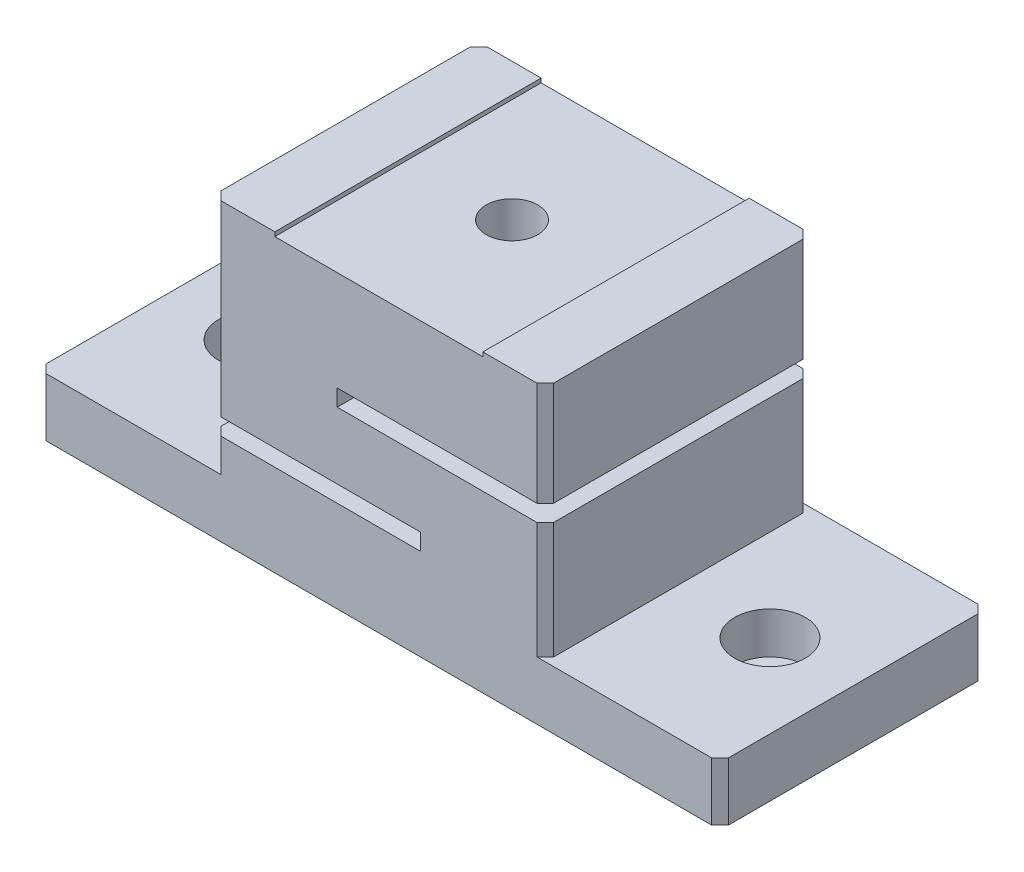
SolidWorks part; units mm, degrees
ref_plane "Front Plane" through (0, 0, 0) normal (0, 0, 1) x (1, 0, 0)
ref_plane "Top Plane" through (0, 0, 0) normal (0, 1, 0) x (1, 0, 0)
ref_plane "Right Plane" through (0, 0, 0) normal (1, 0, 0) x (0, 0, -1)
sketch "Sketch1" plane through (0, 0, 0) normal (0, 1, 0) x (1, 0, 0)
  line L1 (-41, -16) -> (41, -16)
  line L2 (-41, -16) -> (-41, 16)
  line L3 (-41, 16) -> (41, 16)
  line L4 (41, -16) -> (41, 16)
  line L5 (-41, -16) -> (41, 16) construction
  line L6 (-41, 16) -> (41, -16) construction
  point P0 (0, 0)
  dimension "D1" = 82
  dimension "D2" = 32
extrude "Boss-Extrude1" add sketch "Sketch1" along normal blind 7
sketch "Sketch2" plane through (0, 7, 0) normal (0, 1, 0) x (1, 0, 0)
  line L0 (41, 16) -> (-41, 16) construction
  line L1 (-20, -16) -> (20, -16)
  line L2 (-20, -16) -> (-20, 16)
  line L3 (-20, 16) -> (20, 16)
  line L4 (20, -16) -> (20, 16)
  line L5 (-20, -16) -> (20, 16) construction
  line L6 (-20, 16) -> (20, -16) construction
  point P0 (0, 0)
  dimension "D1" = 40
extrude "Boss-Extrude2" add sketch "Sketch2" along normal blind 28.5
sketch "Sketch3" plane through (0, 7, 0) normal (0, 1, 0) x (1, 0, 0)
  line L0 (20, -16) -> (41, -16) construction
  line L1 (41, -16) -> (41, 16) construction
  line L2 (-41, -16) -> (-20, -16) construction
  line L3 (-41, 16) -> (-41, -16) construction
  circle A0 centre (31, 0) radius 2.1
  circle A1 centre (-31, 0) radius 2.1
  dimension "D1" = 4.2
  dimension "D2" = 4.2
  dimension "D3" = 16
  dimension "D4" = 10
  dimension "D5" = 16
  dimension "D6" = 10
extrude "Cut-Extrude1" cut sketch "Sketch3" against normal blind 28.5
sketch "Sketch4" plane through (0, 7, 0) normal (0, 1, 0) x (1, 0, 0)
  circle A0 centre (-31, 0) radius 4.25
  circle A1 centre (31, 0) radius 4.25
  dimension "D1" = 8.5
  dimension "D2" = 8.5
extrude "Cut-Extrude2" cut sketch "Sketch4" against normal blind 5
sketch "Sketch5" plane through (0, 0, -16) normal (0, 0, -1) x (-1, 0, 0)
  line L0 (20, 35.5) -> (20, 7) construction
  line L1 (-5, 13) -> (45, 13)
  line L2 (-5, 13) -> (-5, 11)
  line L3 (-5, 11) -> (45, 11)
  line L4 (45, 13) -> (45, 11)
  line L5 (-5, 13) -> (45, 11) construction
  line L6 (-5, 11) -> (45, 13) construction
  line L7 (20, 7) -> (41, 7) construction
  line L8 (-20, 35.5) -> (-20, 7) construction
  line L9 (5, 21) -> (-45, 21)
  line L10 (5, 21) -> (5, 23)
  line L11 (5, 23) -> (-45, 23)
  line L12 (-45, 21) -> (-45, 23)
  line L13 (5, 21) -> (-45, 23) construction
  line L14 (5, 23) -> (-45, 21) construction
  line L15 (-41, 7) -> (-20, 7) construction
  line L16 (-20, 35.5) -> (20, 35.5) construction
  line L17 (12.5, 35) -> (-12.5, 35)
  line L18 (12.5, 35) -> (12.5, 36)
  line L19 (12.5, 36) -> (-12.5, 36)
  line L20 (-12.5, 35) -> (-12.5, 36)
  line L21 (12.5, 35) -> (-12.5, 36) construction
  line L22 (12.5, 36) -> (-12.5, 35) construction
  point P0 (20, 12)
  point P9 (-20, 22)
  point P18 (0, 35.5)
  dimension "D1" = 2
  dimension "D2" = 5
  dimension "D3" = 25
  dimension "D4" = 2
  dimension "D5" = 25
  dimension "D6" = 15
  dimension "D7" = 1
  dimension "D8" = 25
extrude "Cut-Extrude3" cut sketch "Sketch5" against normal blind 75
sketch "Sketch6" plane through (0, 0, 0) normal (0, -1, 0) x (1, 0, 0)
  circle A0 centre (0, 0) radius 6.5
  dimension "D1" = 13
extrude "Cut-Extrude4" cut sketch "Sketch6" against normal blind 30
sketch "Sketch7" plane through (0, 30, 0) normal (0, -1, 0) x (1, 0, 0)
  circle A0 centre (0, 0) radius 3.1
  dimension "D1" = 6.2
extrude "Cut-Extrude5" cut sketch "Sketch7" against normal blind 30
chamfer "Chamfer1" distance 1 angle 45 12 edges at (20, 29.25, 16) (20, 14, 16) (20, 29.25, -16) (20, 14, -16) (-20, 9, 16) (-20, 24.25, 16) (-20, 24.25, -16) (-20, 9, -16) (41, 3.5, 16) (41, 3.5, -16) (-41, 3.5, 16) (-41, 3.5, -16)
